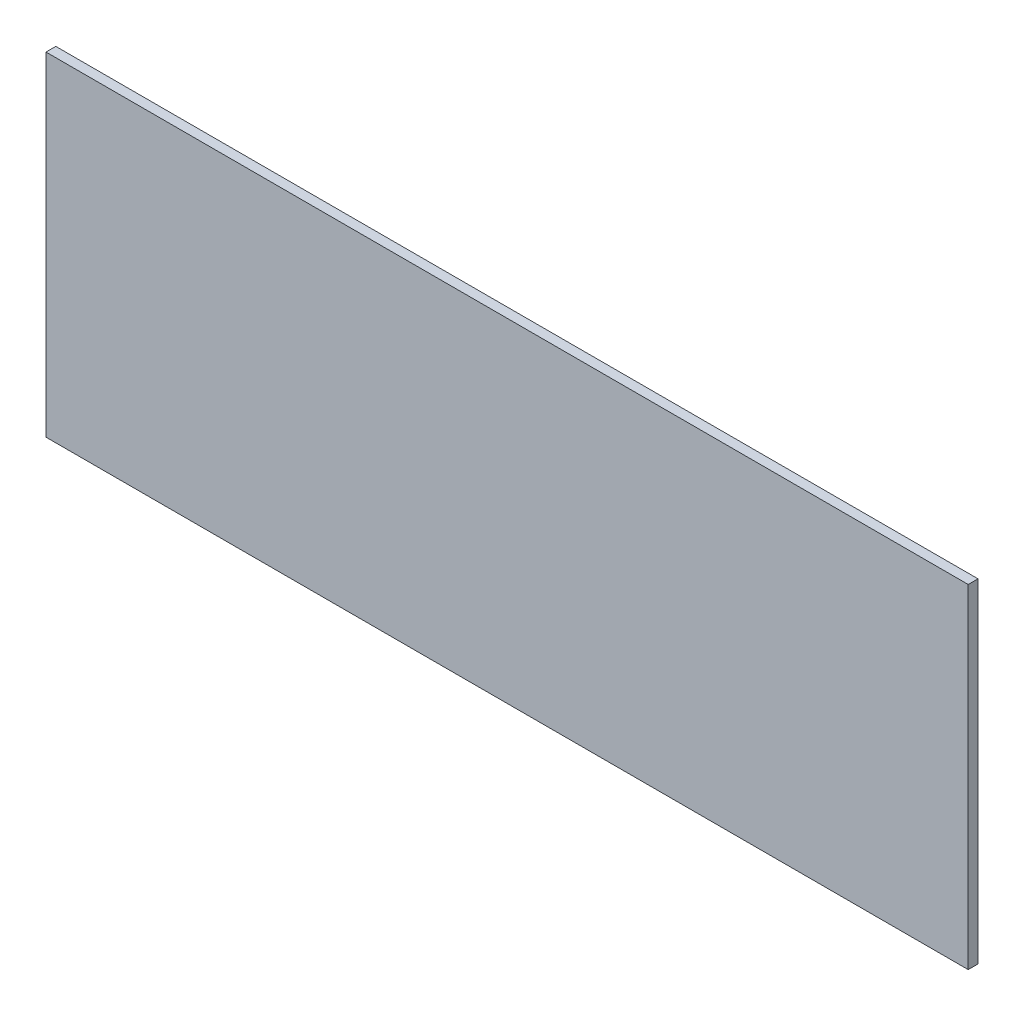
SolidWorks part; units mm, degrees
ref_plane "前视基准面" through (0, 0, 0) normal (0, 0, 1) x (1, 0, 0)
ref_plane "上视基准面" through (0, 0, 0) normal (0, 1, 0) x (1, 0, 0)
ref_plane "右视基准面" through (0, 0, 0) normal (1, 0, 0) x (0, 0, -1)
sketch "草图1" plane through (0, 0, 0) normal (0, 0, 1) x (1, 0, 0)
  line L0 (0, 0) -> (0, 170)
  line L1 (0, 170) -> (470, 170)
  line L2 (470, 170) -> (470, 0)
  line L3 (470, 0) -> (0, 0)
extrude "凸台-拉伸1" add sketch "草图1" along normal blind 5
